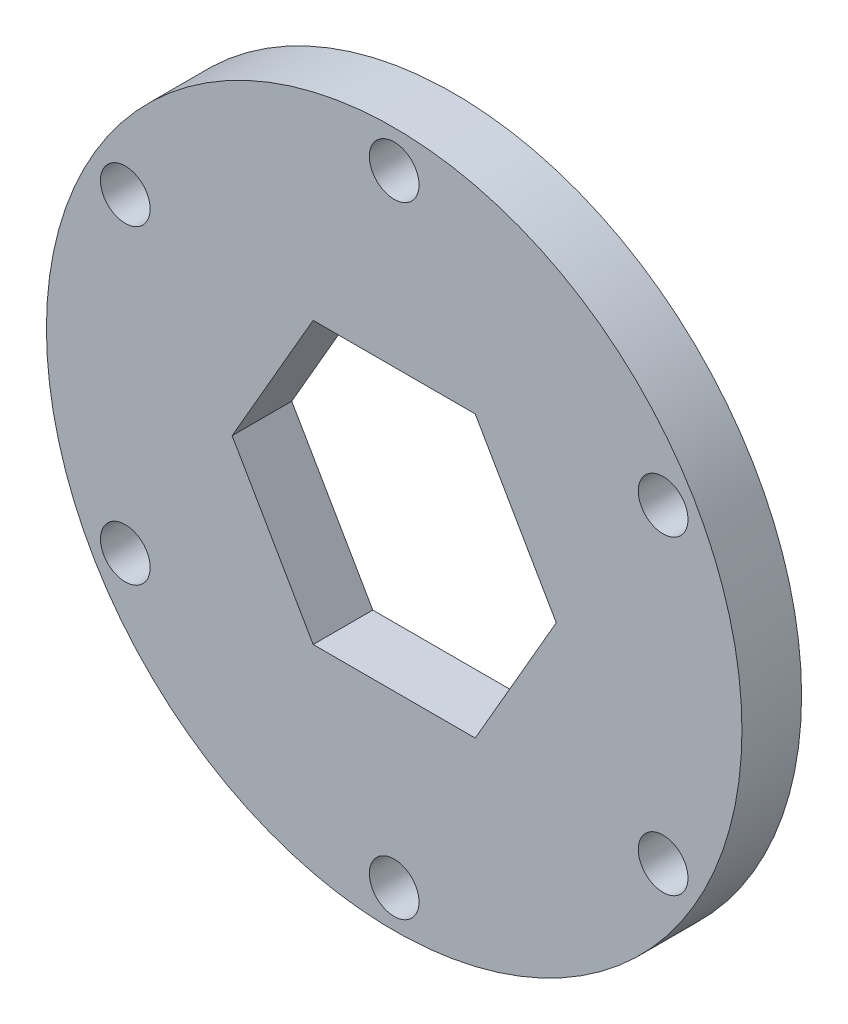
from build123d import *

# Parameters (mm, degrees)
SKETCH1_R           = 70
SKETCH1_R_2         = 5
BOSS_EXTRUDE1_DEPTH = 12


with BuildPart() as part:
    # Sketch1 → Boss-Extrude1 (new body)
    with BuildSketch(Plane.XY):
        Circle(SKETCH1_R)
        with Locations((0, 62.5)):
            Circle(SKETCH1_R_2, mode=Mode.SUBTRACT)
        with Locations((54.126587737, 31.25)):
            Circle(SKETCH1_R_2, mode=Mode.SUBTRACT)
        with Locations((54.126587737, -31.25)):
            Circle(SKETCH1_R_2, mode=Mode.SUBTRACT)
        with Locations((0, -62.5)):
            Circle(SKETCH1_R_2, mode=Mode.SUBTRACT)
        with Locations((-54.126587737, -31.25)):
            Circle(SKETCH1_R_2, mode=Mode.SUBTRACT)
        with Locations((-54.126587737, 31.25)):
            Circle(SKETCH1_R_2, mode=Mode.SUBTRACT)
        Polygon((32.620290209, 0), (16.310145105, 28.25), (-16.310145105, 28.25), (-32.620290209, 0), (-16.310145105, -28.25), (16.310145105, -28.25), align=None, mode=Mode.SUBTRACT)
    extrude(amount=BOSS_EXTRUDE1_DEPTH)


solid = part.part
